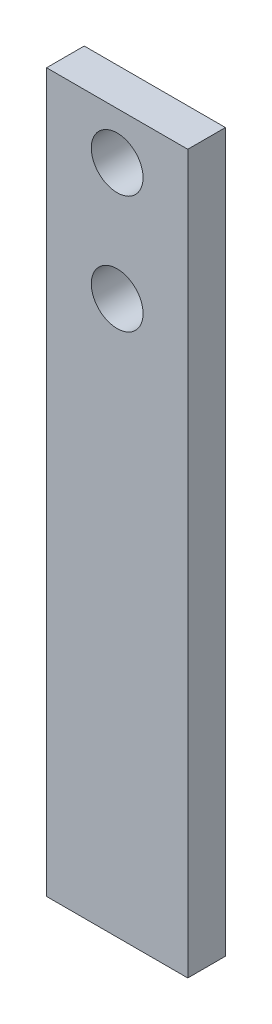
SolidWorks part; units mm, degrees
material "A3"
ref_plane "前视基准面" through (0, 0, 0) normal (0, 0, 1) x (1, 0, 0)
ref_plane "上视基准面" through (0, 0, 0) normal (0, 1, 0) x (1, 0, 0)
ref_plane "右视基准面" through (0, 0, 0) normal (1, 0, 0) x (0, 0, -1)
sketch "草图1" plane through (0, 0, 0) normal (0, 0, 1) x (1, 0, 0)
  line L1 (-30, -152.5) -> (30, -152.5)
  line L2 (-30, -152.5) -> (-30, 152.5)
  line L3 (-30, 152.5) -> (30, 152.5)
  line L4 (30, -152.5) -> (30, 152.5)
  line L5 (-30, -152.5) -> (30, 152.5) construction
  line L6 (-30, 152.5) -> (30, -152.5) construction
  circle A0 centre (0, 132.5) radius 11
  circle A1 centre (0, 82.5) radius 11
  point P0 (0, 0)
  dimension "D3" = 22
  dimension "D4" = 20
  dimension "D1" = 305
  dimension "D2" = 60
  dimension "D5" = 50
extrude "凸台-拉伸1" add sketch "草图1" along normal mid plane 16
